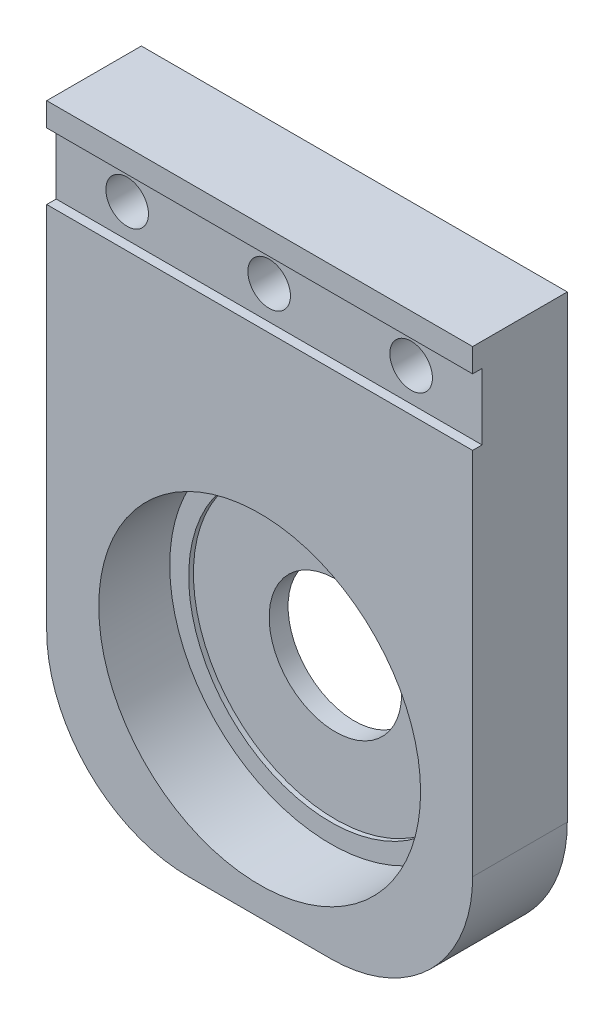
from build123d import *

# Parameters (mm, degrees)
SKETCH1_W                                            = 90
SKETCH1_H                                            = 120
BOSS_EXTRUDE1_DEPTH                                  = 20
SKETCH2_R                                            = 34
CUT_EXTRUDE1_DEPTH                                   = 15
SKETCH3_R                                            = 30
CUT_EXTRUDE2_DEPTH                                   = 1
SKETCH4_R                                            = 14
CUT_EXTRUDE3_DEPTH                                   = 10
MOVE_FACE1_BY                                        = 2.02
FILLET1_R                                            = 30
MOVE_FACE2_BY                                        = 5
CBORE_FOR_M8_HEXAGON_SOCKET_HEAD_CAP_SCR_D           = 9
CBORE_FOR_M8_HEXAGON_SOCKET_HEAD_CAP_SCR_DEPTH       = 80.25
CBORE_FOR_M8_HEXAGON_SOCKET_HEAD_CAP_SCR_CBORE_D     = 15
CBORE_FOR_M8_HEXAGON_SOCKET_HEAD_CAP_SCR_CBORE_DEPTH = 9
CBORE_FOR_M8_HEXAGON_SOCKET_HEAD_CAP_SCR_TIP         = 2.703872786
SKETCH7_W                                            = 90
SKETCH7_H                                            = 14
CUT_EXTRUDE4_DEPTH                                   = 2


with BuildPart() as part:
    # Sketch1 → Boss-Extrude1 (new body)
    with BuildSketch(Plane.XY):
        Rectangle(SKETCH1_W, SKETCH1_H)
    extrude(amount=BOSS_EXTRUDE1_DEPTH)

    # Sketch2 → Cut-Extrude1 (cut)
    with BuildSketch(Plane.XY.offset(20)):
        with Locations((0, -20)):
            Circle(SKETCH2_R)
    extrude(amount=-CUT_EXTRUDE1_DEPTH, mode=Mode.SUBTRACT)

    # Sketch3 → Cut-Extrude2 (cut)
    with BuildSketch(Plane.XY.offset(5)):
        with Locations((0, -20)):
            Circle(SKETCH3_R)
    extrude(amount=-CUT_EXTRUDE2_DEPTH, mode=Mode.SUBTRACT)

    # Sketch4 → Cut-Extrude3 (cut)
    with BuildSketch(Plane.XY.offset(4)):
        with Locations((0, -20)):
            Circle(SKETCH4_R)
    extrude(amount=-CUT_EXTRUDE3_DEPTH, mode=Mode.SUBTRACT)

    # Move Face1: a face moved outward by 2.02
    extrude(part.faces().sort_by_distance((0, 60, 10))[0], amount=MOVE_FACE1_BY, dir=(0, 1, 0))

    # Fillet1
    fillet1_edges = [part.edges().sort_by_distance(p)[0] for p in [
        (45, -60, 10),
        (-45, -60, 10),
    ]]
    fillet(fillet1_edges, radius=FILLET1_R)

    # Move Face2: a face moved outward by 5.0
    extrude(part.faces().sort_by_distance((0, 62.02, 10))[0], amount=MOVE_FACE2_BY, dir=(0, 1, 0))

    # CBORE for M8 Hexagon socket head cap screws1
    with Locations(Plane(origin=(0, 0, 0), x_dir=(-1, 0, 0), z_dir=(0, 0, -1))):
        with Locations((30, 55.02), (-30, 55.02), (0, 55.02)):
            CounterBoreHole(CBORE_FOR_M8_HEXAGON_SOCKET_HEAD_CAP_SCR_D / 2, CBORE_FOR_M8_HEXAGON_SOCKET_HEAD_CAP_SCR_CBORE_D / 2, CBORE_FOR_M8_HEXAGON_SOCKET_HEAD_CAP_SCR_CBORE_DEPTH, depth=CBORE_FOR_M8_HEXAGON_SOCKET_HEAD_CAP_SCR_DEPTH)
            with Locations((0, 0, -(CBORE_FOR_M8_HEXAGON_SOCKET_HEAD_CAP_SCR_DEPTH + CBORE_FOR_M8_HEXAGON_SOCKET_HEAD_CAP_SCR_TIP / 2))):  # 118° drill point
                Cone(0, CBORE_FOR_M8_HEXAGON_SOCKET_HEAD_CAP_SCR_D / 2, CBORE_FOR_M8_HEXAGON_SOCKET_HEAD_CAP_SCR_TIP, mode=Mode.SUBTRACT)

    # Sketch7 → Cut-Extrude4 (cut)
    with BuildSketch(Plane.XY.offset(20)):
        with Locations((0, 55.02)):
            Rectangle(SKETCH7_W, SKETCH7_H)
    extrude(amount=-CUT_EXTRUDE4_DEPTH, mode=Mode.SUBTRACT)


solid = part.part
